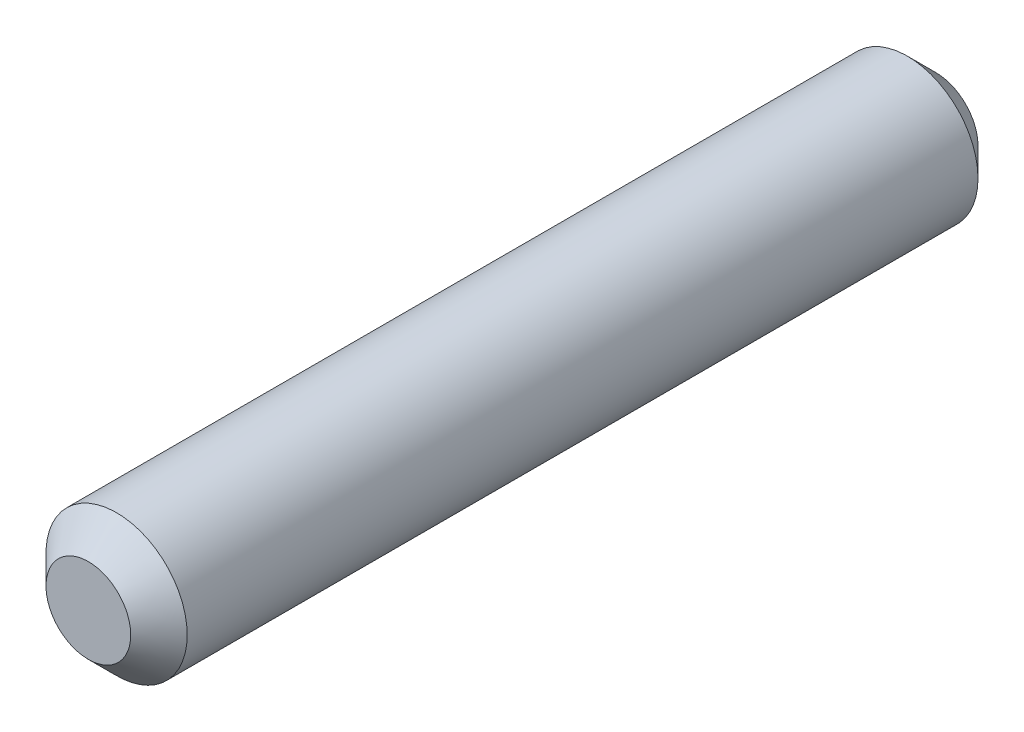
from build123d import *

# Parameters (mm, degrees)
SKETCH1_R           = 2.5
BOSS_EXTRUDE1_DEPTH = 30
CHAMFER1_SIZE       = 1


with BuildPart() as part:
    # Sketch1 → Boss-Extrude1 (new body)
    with BuildSketch(Plane.XY):
        Circle(SKETCH1_R)
    extrude(amount=BOSS_EXTRUDE1_DEPTH)

    # Chamfer1
    chamfer1_edges = [part.edges().sort_by_distance(p)[0] for p in [
        (-2.5, 0, 0),
        (-2.5, 0, 30),
    ]]
    chamfer(chamfer1_edges, length=CHAMFER1_SIZE)


solid = part.part
